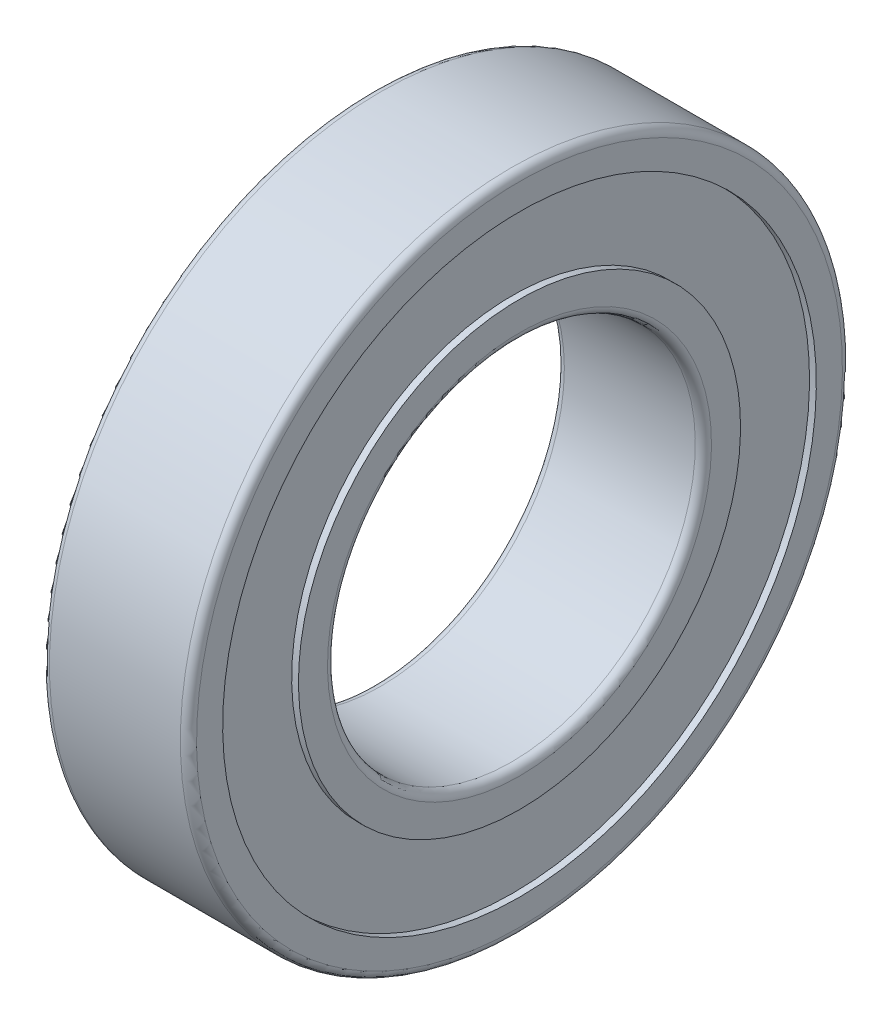
from build123d import *

# Parameters (mm, degrees)
FILLET1_R = 1.1
FILLET2_R = 1.1


with BuildPart() as part:
    # Sketch1 → Revolve1 (revolve)
    with BuildSketch(Plane.XY, mode=Mode.PRIVATE) as revolve1_sk:
        Polygon((0, 25), (20, 25), (20, 30.05), (19.08, 30.05), (19.08, 40.35), (20, 40.35), (20, 45), (0, 45), (0, 40.35), (0.92, 40.35), (0.92, 30.05), (0, 30.05), align=None)
    revolve(revolve1_sk.sketch.rotate(Axis((0, 0, 0), (1, 0, 0)), 180), axis=Axis((0, 0, 0), (1, 0, 0)))

    # Fillet1
    fillet1_edges = [part.edges().sort_by_distance(p)[0] for p in [
        (0, 45, 0),
        (20, 45, 0),
    ]]
    fillet(fillet1_edges, radius=FILLET1_R)

    # Fillet2
    fillet2_edges = [part.edges().sort_by_distance(p)[0] for p in [
        (20, 25, 0),
        (0, 25, 0),
    ]]
    fillet(fillet2_edges, radius=FILLET2_R)


solid = part.part
